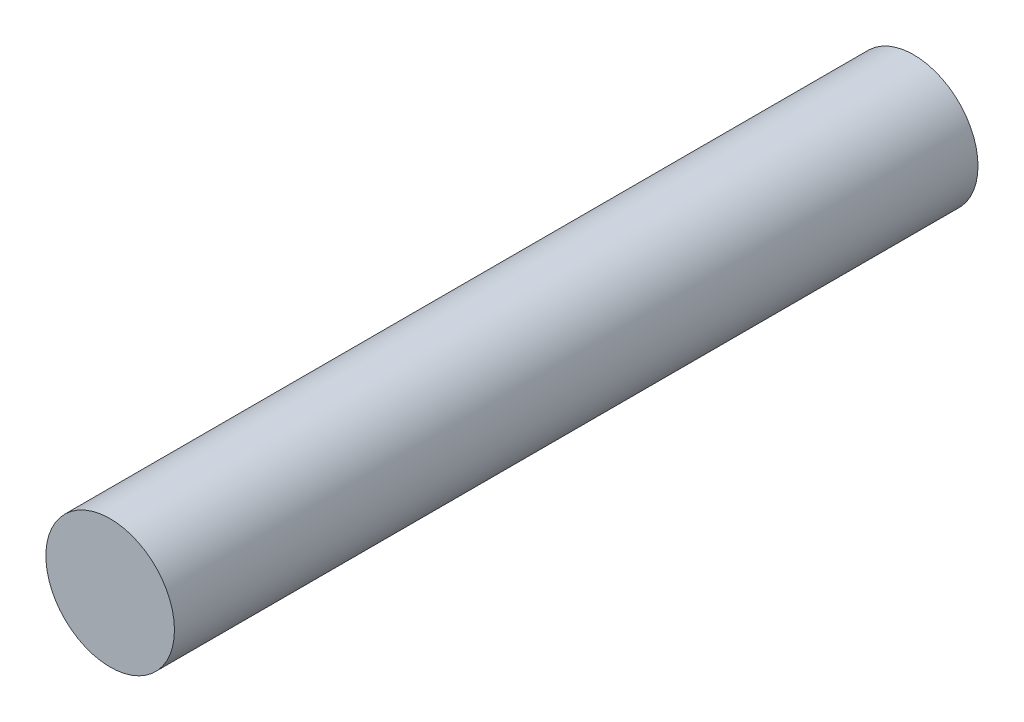
from build123d import *

# Parameters (mm, degrees)
SKETCH_1_R      = 6
EXTRUDE_1_DEPTH = 37.5


with BuildPart() as part:
    # 草图1 → 凸台-拉伸1 (new, symmetric)
    with BuildSketch(Plane.XY):
        Circle(SKETCH_1_R)
    extrude(amount=EXTRUDE_1_DEPTH, both=True)


solid = part.part
